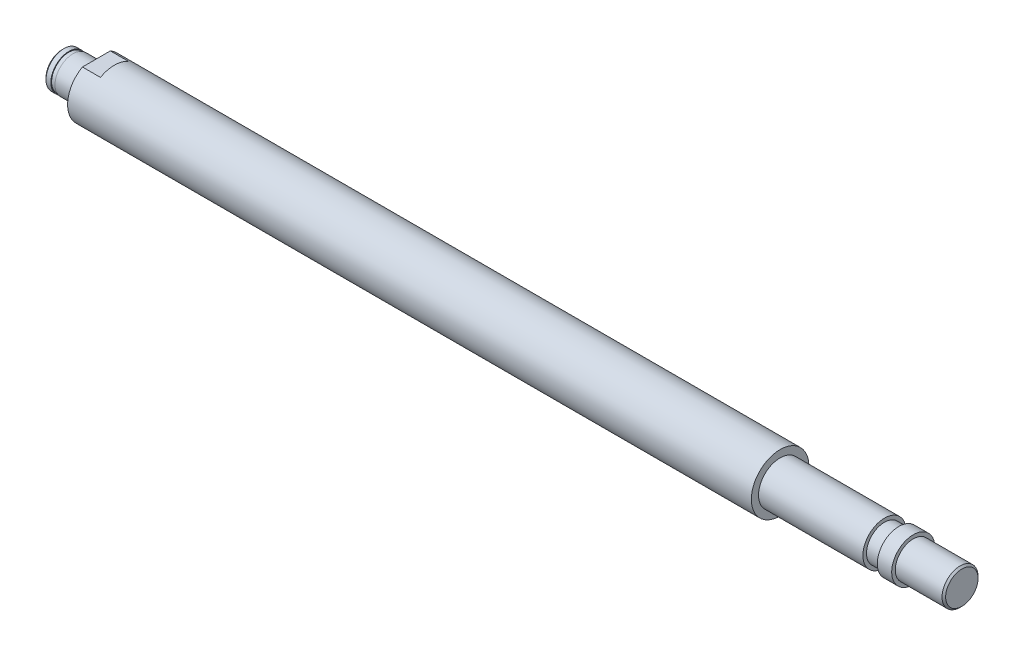
SolidWorks part; units mm, degrees
material "SCM450"
ref_plane "Front Plane" through (0, 0, 0) normal (0, 0, 1) x (1, 0, 0)
ref_plane "Top Plane" through (0, 0, 0) normal (0, 1, 0) x (1, 0, 0)
ref_plane "Right Plane" through (0, 0, 0) normal (1, 0, 0) x (0, 0, -1)
sketch "Sketch1" plane through (0, 0, 0) normal (0, 0, 1) x (1, 0, 0)
  line L0 (0, 0) -> (83.6379, 0) construction
  line L1 (0, 0) -> (0, 5)
  line L2 (0, 5) -> (1.85, 5)
  line L3 (1.85, 5) -> (1.85, 4.8)
  line L4 (1.85, 4.8) -> (3, 4.8)
  line L5 (3, 4.8) -> (3, 5)
  line L6 (3, 5) -> (9.5, 5)
  line L7 (9.5, 5) -> (9.5, 8)
  line L8 (9.5, 8) -> (199.5, 8)
  line L9 (199.5, 8) -> (199.5, 6)
  line L10 (199.5, 6) -> (228.5, 6)
  line L11 (228.5, 6) -> (228.5, 5)
  line L12 (228.5, 5) -> (232.5, 5)
  line L13 (232.5, 5) -> (232.5, 6)
  line L14 (232.5, 6) -> (236.5, 6)
  line L15 (250, 5) -> (250, 0)
  line L16 (250, 0) -> (0, 0)
  line L17 (236.5, 6) -> (236.5, 5)
  line L18 (236.5, 5) -> (250, 5)
  dimension "D1" = 5
  dimension "D2" = 4.8
  dimension "D3" = 5
  dimension "D4" = 8
  dimension "D5" = 3
  dimension "D6" = 1.15
  dimension "D7" = 6.5
  dimension "D8" = 250
  dimension "D9" = 13.5
  dimension "D10" = 6
  dimension "D11" = 5
  dimension "D12" = 6
  dimension "D13" = 5
  dimension "D14" = 29
  dimension "D15" = 4
  dimension "D16" = 4
revolve "Revolve1" add sketch "Sketch1" angle 360 about L0
cosmetic thread "Cosmetic Thread1" parameters "D1"=13, "D2"=10.647
cosmetic thread "Cosmetic Thread2" parameters "D1"=6, "D2"=10.647
cosmetic thread "Cosmetic Thread3" parameters "D1"=6, "D2"=10.647
sketch "Sketch2" plane through (9.5, 0, 0) normal (-1, 0, 0) x (0, 0, 1)
  line L1 (-11.4852, -7) -> (11.4852, -7)
  line L2 (-11.4852, -7) -> (-11.4852, 7)
  line L3 (-11.4852, 7) -> (11.4852, 7)
  line L4 (11.4852, -7) -> (11.4852, 7)
  line L5 (-11.4852, -7) -> (11.4852, 7) construction
  line L6 (-11.4852, 7) -> (11.4852, -7) construction
  point P0 (0, 0)
  dimension "D1" = 14
extrude "Cut-Extrude1" cut sketch "Sketch2" against normal blind 5 flip side to cut
chamfer "Chamfer1" distance 0.5 angle 45 2 edges at (250, 0, 5) (0, 0, 5)
